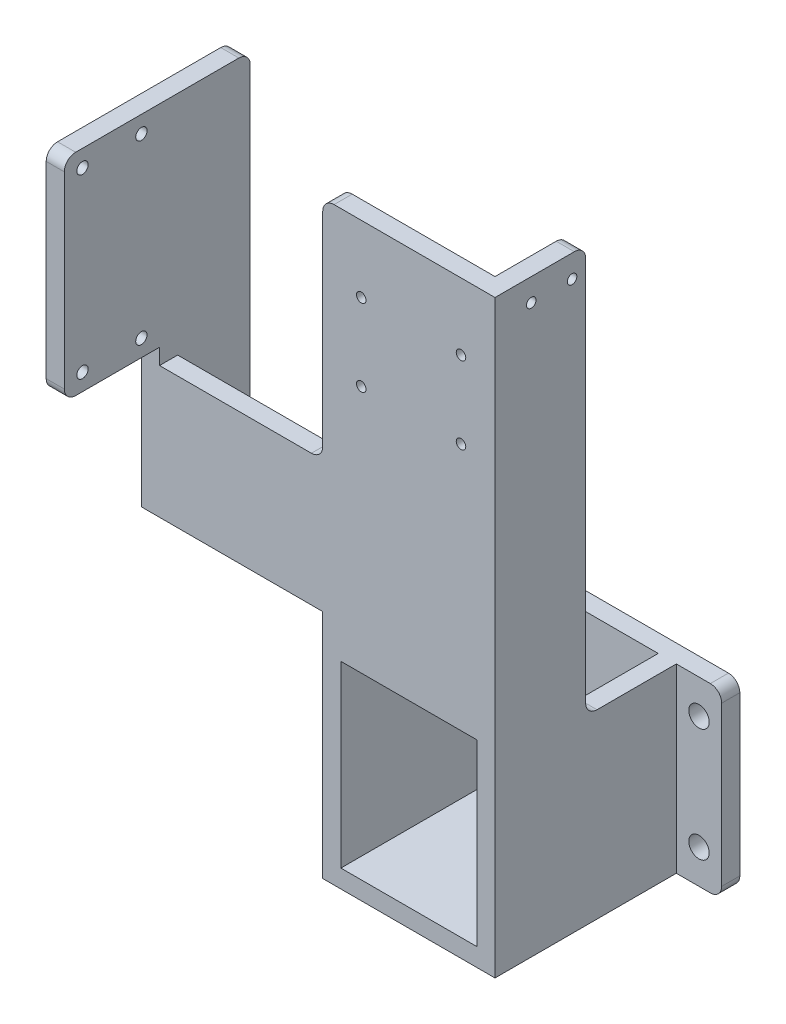
from build123d import *

# Parameters (mm, degrees)
SKETCH_1_W             = 116
SKETCH_1_H             = 80
EXTRUDE_1_DEPTH        = 8
SKETCH_2_W             = 8
SKETCH_2_H             = 80
EXTRUDE_2_DEPTH        = 80
SKETCH_4_W             = 8
SKETCH_4_H             = 40
EXTRUDE_3_DEPTH        = 180
SKETCH_5_W             = 60
SKETCH_5_H             = 8
EXTRUDE_4_DEPTH        = 80
SKETCH_8_W             = 8
SKETCH_8_H             = 40
EXTRUDE_7_DEPTH        = 30
SKETCH_10_W            = 40
SKETCH_10_H            = 8
EXTRUDE_8_DEPTH        = 80
SKETCH_11_W            = 8
SKETCH_11_H            = 40
EXTRUDE_9_DEPTH        = 150
SKETCH_12_W            = 8
SKETCH_12_H            = 93
EXTRUDE_10_DEPTH       = 68
SKETCH_14_W            = 8
SKETCH_14_H            = 93
EXTRUDE_12_DEPTH       = 42
FILLET_1_R             = 5
FILLET_2_R             = 5
HOLE_WIZARD_9_0_9_1_D  = 9
HOLE_WIZARD_M5_1_D     = 4.2
HOLE_WIZARD_M6_1_D     = 5
HOLE_WIZARD_M5_2_D     = 4.2
HOLE_WIZARD_M5_2_DEPTH = 10.4
HOLE_WIZARD_M5_2_TIP   = 1.2618073
EXTRUDE_15_DEPTH       = 8
FILLET_3_R             = 5


with BuildPart() as part:
    # 草图1 → 凸台-拉伸1 (new body)
    with BuildSketch(Plane.XY):
        with Locations((58, 40)):
            Rectangle(SKETCH_1_W, SKETCH_1_H)
    extrude(amount=EXTRUDE_1_DEPTH)

    # 草图2 → 凸台-拉伸2 (add)
    with BuildSketch(Plane.XY.offset(8)):
        with Locations((24, 40)):
            Rectangle(SKETCH_2_W, SKETCH_2_H)
        with Locations((92, 40)):
            Rectangle(SKETCH_2_W, SKETCH_2_H)
    extrude(amount=EXTRUDE_2_DEPTH)

    # 草图4 → 凸台-拉伸3 (add)
    with BuildSketch(Plane(origin=(0, 80, 0), x_dir=(1, 0, 0), z_dir=(0, 1, 0))):
        with Locations((92, -68)):
            Rectangle(SKETCH_4_W, SKETCH_4_H)
    extrude(amount=EXTRUDE_3_DEPTH)

    # 草图5 → 凸台-拉伸4 (add)
    with BuildSketch(Plane.XY.offset(8)):
        with Locations((58, 4)):
            Rectangle(SKETCH_5_W, SKETCH_5_H)
    extrude(amount=EXTRUDE_4_DEPTH)

    # 草图8 → 凸台-拉伸7 (add)
    with BuildSketch(Plane(origin=(0, 80, 0), x_dir=(1, 0, 0), z_dir=(0, 1, 0))):
        with Locations((24, -68)):
            Rectangle(SKETCH_8_W, SKETCH_8_H)
    extrude(amount=EXTRUDE_7_DEPTH)

    # 草图10 → 凸台-拉伸8 (add)
    with BuildSketch(Plane.ZY.offset(-20)):
        with Locations((68, 106)):
            Rectangle(SKETCH_10_W, SKETCH_10_H)
    extrude(amount=EXTRUDE_8_DEPTH)

    # 草图11 → 凸台-拉伸9 (add)
    with BuildSketch(Plane(origin=(0, 110, 0), x_dir=(1, 0, 0), z_dir=(0, 1, 0))):
        with Locations((-56, -68)):
            Rectangle(SKETCH_11_W, SKETCH_11_H)
    extrude(amount=EXTRUDE_9_DEPTH)

    # 草图12 → 凸台-拉伸10 (add)
    with BuildSketch(Plane.ZY.offset(-88)):
        with Locations((84, 213.5)):
            Rectangle(SKETCH_12_W, SKETCH_12_H)
    extrude(amount=EXTRUDE_10_DEPTH)

    # 草图14 → 凸台-拉伸12 (add)
    with BuildSketch(Plane.XY.offset(88)):
        with Locations((-56, 213.5)):
            Rectangle(SKETCH_14_W, SKETCH_14_H)
    extrude(amount=EXTRUDE_12_DEPTH)

    # 圆角1
    fillet_1_edges = [part.edges().sort_by_distance(p)[0] for p in [
        (-56, 260, 48),
        (24, 80, 48),
        (92, 80, 48),
        (92, 260, 48),
        (-56, 260, 130),
        (-56, 167, 130),
        (20, 260, 84),
    ]]
    fillet(fillet_1_edges, radius=FILLET_1_R)

    # 圆角2
    fillet_2_edges = [part.edges().sort_by_distance(p)[0] for p in [
        (0, 80, 4),
        (0, 0, 4),
        (116, 80, 4),
        (116, 0, 4),
    ]]
    fillet(fillet_2_edges, radius=FILLET_2_R)

    # Ø9.0 (9) 直径孔1 (through all)
    with Locations(Plane.XY.offset(8)):
        with Locations((106, 15), (106, 65)):
            hole_wizard_9_0_9_1 = Hole(HOLE_WIZARD_9_0_9_1_D / 2)

    # 镜向1: Ø9.0 (9) 直径孔1 across plane
    add(hole_wizard_9_0_9_1.mirror(Plane(origin=(58, 0, 0), x_dir=(0, 0, 1), z_dir=(1, 0, 0))), mode=Mode.SUBTRACT)

    # M5 螺纹孔1 (through all)
    with Locations(Plane.XY.offset(88)):
        with Locations((37, 196.5), (81, 196.5), (81, 230.5), (37, 230.5)):
            Hole(HOLE_WIZARD_M5_1_D / 2)

    # M6 螺纹孔1 (through all)
    with Locations(Plane(origin=(-52, 0, 0), x_dir=(0, 0, -1), z_dir=(1, 0, 0))):
        with Locations((-96, 252.5), (-122, 252.5), (-122, 174.5), (-96, 174.5)):
            Hole(HOLE_WIZARD_M6_1_D / 2)

    # M5 螺纹孔2
    with Locations(Plane(origin=(96, 0, 0), x_dir=(0, 0, -1), z_dir=(1, 0, 0))):
        with Locations((-72, 250), (-54, 250)):
            Hole(HOLE_WIZARD_M5_2_D / 2, depth=HOLE_WIZARD_M5_2_DEPTH)
            with Locations((0, 0, -(HOLE_WIZARD_M5_2_DEPTH + HOLE_WIZARD_M5_2_TIP / 2))):  # 118° drill point
                Cone(0, HOLE_WIZARD_M5_2_D / 2, HOLE_WIZARD_M5_2_TIP, mode=Mode.SUBTRACT)

    # 草图27 → 凸台-拉伸15 (add)
    with BuildSketch(Plane.XY.offset(88)):
        Polygon((88, 87), (88, 167), (20, 167), (20, 160), (-52, 160), (-52, 110), (28, 110), (28, 87), align=None)
    extrude(amount=-EXTRUDE_15_DEPTH)

    # 圆角3
    fillet_3_edges = [part.edges().sort_by_distance(p)[0] for p in [
        (20, 160, 84),
    ]]
    fillet(fillet_3_edges, radius=FILLET_3_R)


solid = part.part
